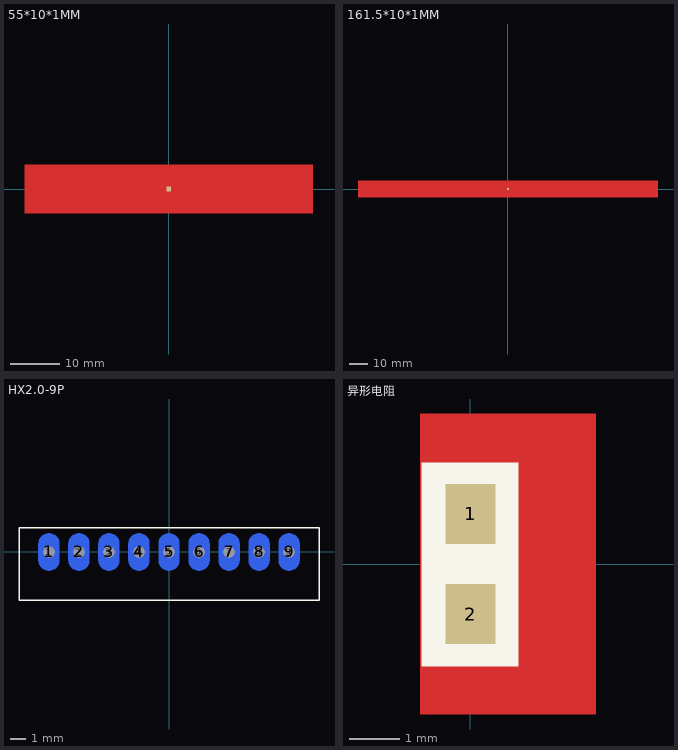
[diagram p0: the footprints below, top view; thin cyan lines are the x and y axes]
# Altium footprint library MISC89348.PcbLib: 4 footprints
Each footprint in its own frame and in the unit in brackets; x right, y up, seen from the top. Pads: shape width x height; smd on the part's side, far side on the other; paste and mask are expansions set on the pad; w line width, h text height; cw(c..) or ccw(c..) is an arc to the next point about the centre after c.

## 55*10*1MM [mm]
pads (1):
  rect 1x1 smd: 1(0,0)
Top Layer:
  rectangle: -29.499,-5 29.501,5
Top Solder:
  region: 24.049,4.919 24.049,-4.982 27.479,-4.982 27.479,4.919
  rectangle: -27.4,2.15 27.45,4.95
  rectangle: -27.45,-4.95 27.45,-2.15
  region: -27.45,4.887 -27.45,-4.95 -23.97,-4.95 -23.97,4.887
  region: -2.1,4.9 -2.1,-4.949 2.1,-4.949 2.1,4.9

## 161.5*10*1MM [mm]
pads (1):
  rect 1x1 smd: 1(0,0)
Top Layer:
  rectangle: -82.749,-4.7 82.751,4.7
Top Solder:
  region: -80.7,4.587 -80.7,-4.65 -75.22,-4.65 -75.22,4.587
  rectangle: -80.7,2.15 80.7,4.587
  region: 75.299,4.59 75.299,-4.64 80.729,-4.64 80.729,4.59
  rectangle: -80.7,-4.65 80.65,-2.15
  region: -2.1,4.58 -2.1,-4.65 2.1,-4.65 2.1,4.58
  region: -42.475,4.572 -42.475,-4.65 -38.275,-4.65 -38.275,4.572
  region: 38.275,4.6 38.275,-4.64 42.475,-4.64 42.475,4.6

## HX2.0-9P [mm]
pads (18):
  oval 1.4x2.5 smd far side: 1(-8,0) 2(-6,0) 3(-4,0) 4(-2,0) 5(0,0) 6(2,0) 7(4,0) 8(6,0) 9(8,0)
  round 0.75 hole 0.75: 1(-8,0) 2(-6,0) 3(-4,0) 4(-2,0) 5(0,0) 6(2,0) 7(4,0) 8(6,0) 9(8,0)
Top Overlay:
  lines w0.1: -10,-3.2 10,-3.2 10,1.6 -10,1.6 -10,-3.2
Keep-Out Layer:
  drawing of 9 lines, arcs and shapes, not listed
Keep-Out Layer:
  circle w0.01: c0,0 r0.375
  circle w0.01: c2,0 r0.375
  circle w0.01: c4,0 r0.375
  circle w0.01: c6,0 r0.375
  circle w0.01: c8,0 r0.375
  circle w0.01: c-2,0 r0.375
  circle w0.01: c-4,0 r0.375
  circle w0.01: c-6,0 r0.375
  circle w0.01: c-8,0 r0.375

## 异形电阻 [mm]
pads (2):
  rect 1x1.2 smd mask+0: 1(0,1) 2(0,-1)
Top Layer:
  pour cut-out: -1,3 2.5,3 2.5,-3 -1,-3
  region: 0.5,0.125 0.5,2.55 0.5,2.575 0.481,2.621 0.446,2.656 0.4,2.675 0.375,2.675 -0.425,2.675 -0.44,2.675 -0.467,2.664 -0.489,2.642 -0.5,2.615 -0.5,2.6 -0.5,0.125
  region: -0.5,-2.625 -0.5,-2.635 -0.492,-2.653 -0.478,-2.667 -0.46,-2.675 -0.45,-2.675 0.4,-2.675 0.42,-2.675 0.457,-2.66 0.485,-2.632 0.5,-2.595 0.5,-2.575 0.5,-0.125 -0.5,-0.125
  lines w0.2: -0.325,2.5 -0.02,2.5 0,2.5
  lines w0.35: -0.325,-2.5 0,-2.5 1.525,-2.5 ccw(c1.525,-2) 1.525,-1.5 ; -0.325,2.5 -0.02,2.5 0,2.5 1.525,2.5 cw(c1.525,2) 1.525,1.5 ; 1.5,-1.5 cw(c1.5,-1) 1.5,-0.5 ; 1.5,0.5 cw(c1.5,1) 1.5,1.5 ; 1.525,-0.5 ccw(c1.525,0) 1.525,0.5
Top Overlay:
  pour cut-out: 0.955,2.026 -0.979,2.026 -0.979,-2.044 0.955,-2.044
  lines w0.127: -0.762,-0.508 -0.762,-1.778 0.762,-1.778 0.762,-0.508 ; -0.762,0.508 -0.762,1.778 0.762,1.778 0.762,0.508
Top Solder:
  region: 0.5,0.625 0,0.125 -0.5,0.625
  region: 0.5,-0.625 0,-0.125 -0.5,-0.625